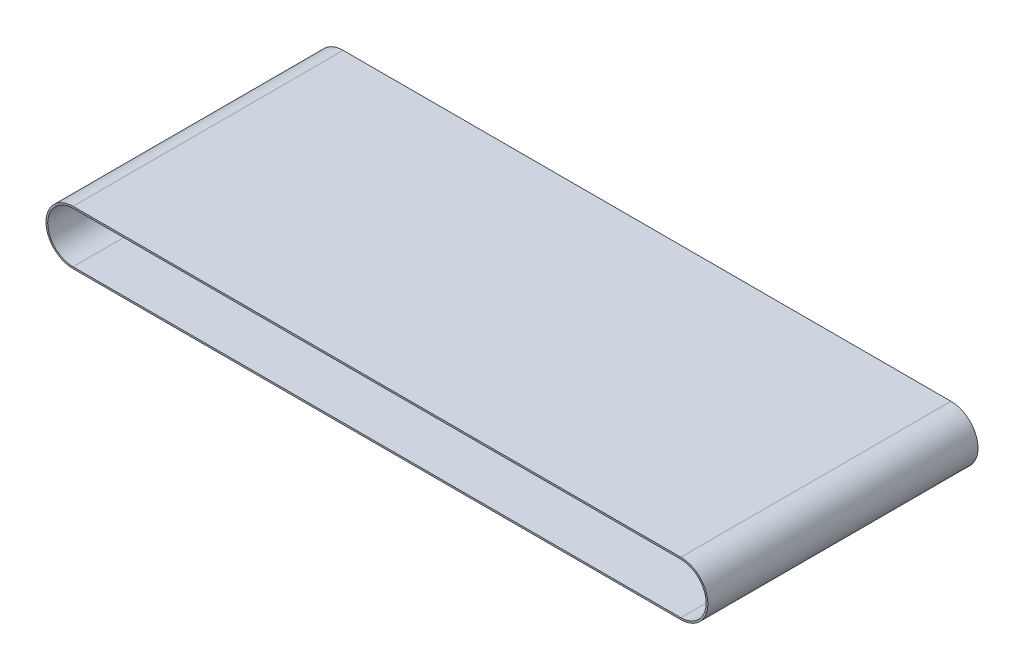
SolidWorks part; units mm, degrees
material "硅橡胶"
ref_plane "前视基准面" through (0, 0, 0) normal (0, 0, 1) x (1, 0, 0)
ref_plane "上视基准面" through (0, 0, 0) normal (0, 1, 0) x (1, 0, 0)
ref_plane "右视基准面" through (0, 0, 0) normal (1, 0, 0) x (0, 0, -1)
sketch "草图1" plane through (0, 0, 0) normal (0, 0, 1) x (1, 0, 0)
  line L0 (0, 0) -> (1800, 0) construction
  line L1 (0, 75) -> (1800, 75)
  line L2 (0, -75) -> (1800, -75)
  arc A0 (0, 75) -> (0, -75) centre (0, 0) ccw
  arc A1 (1800, -75) -> (1800, 75) centre (1800, 0) ccw
  point P3 (900, 0)
  dimension "D2" = 75
  dimension "D1" = 1800
extrude "拉伸-薄壁1" add sketch "草图1" along normal blind 800 thin contours L2 A1 L1 A0 thin type one direction wall 5
